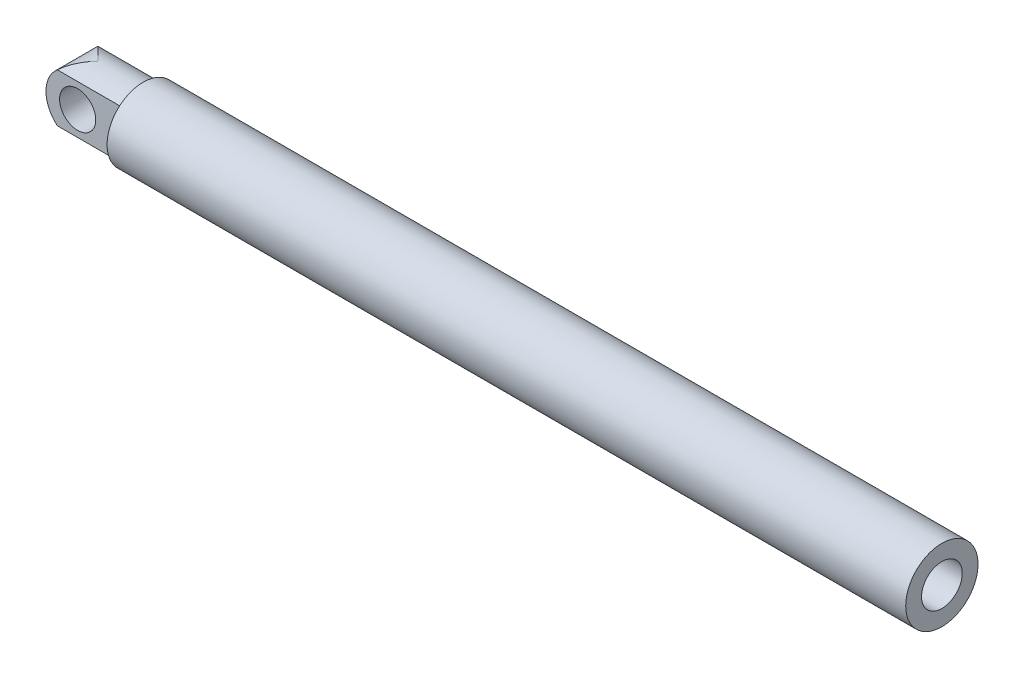
from build123d import *

# Parameters (mm, degrees)
CUT_EXTRUDE_1_DEPTH      = 970.651483782
CUT_EXTRUDE_1_DEPTH_BACK = 970.651483782
SKETCH_2_R               = 20
SKETCH_3_W               = 28.175076561
SKETCH_3_H               = 100
CUT_EXTRUDE_2_DEPTH      = 885.810149128


with BuildPart() as part:
    # Sketch 1 → Revolve 1 (revolve)
    with BuildSketch(Plane.XY, mode=Mode.PRIVATE) as revolve_1_sk:
        Polygon((0, 40), (-883, 40), (-883, 35), (-968, 35), (-968, 0), (-750, 0), (-750, 22.5), (0, 22.5), align=None)
    revolve(revolve_1_sk.sketch.rotate(Axis((-802.16755253, 0, 0), (1, 0, 0)), 90), axis=Axis((-802.16755253, 0, 0), (1, 0, 0)))

    # Sketch 2 → Cut-Extrude 1 (cut, two sides: drawn at the far end of the back side and taken through both)
    with BuildSketch(Plane.XY.offset(-CUT_EXTRUDE_1_DEPTH_BACK)):
        with BuildLine():
            Line((-968, 35), (-968, 0))
            ThreePointArc((-968, 0), (-957.748737342, 24.748737342), (-933, 35))
            Line((-933, 35), (-968, 35))
        make_face()
        with BuildLine():
            Line((-968, 0), (-968, -35))
            Line((-968, -35), (-933, -35))
            ThreePointArc((-933, -35), (-957.748737342, -24.748737342), (-968, 0))
        make_face()
        with Locations((-933, 0)):
            Circle(SKETCH_2_R)
    extrude(amount=CUT_EXTRUDE_1_DEPTH + CUT_EXTRUDE_1_DEPTH_BACK, mode=Mode.SUBTRACT)

    # Sketch 3 → Cut-Extrude 2 (cut, through all)
    with BuildSketch(Plane.ZY.offset(883)):
        with Locations((-36.58753828, 0)):
            Rectangle(SKETCH_3_W, SKETCH_3_H)
        with Locations((36.58753828, 0)):
            Rectangle(SKETCH_3_W, SKETCH_3_H)
    extrude(amount=CUT_EXTRUDE_2_DEPTH, mode=Mode.SUBTRACT)


solid = part.part
